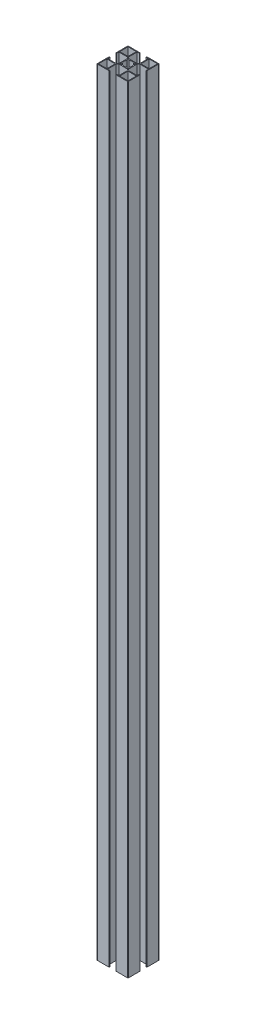
SolidWorks part; units mm, degrees
material "6061 Aluminium alloy"
ref_plane "Front" through (0, 0, 0) normal (0, 0, 1) x (1, 0, 0)
ref_plane "Top" through (0, 0, 0) normal (0, 1, 0) x (1, 0, 0)
ref_plane "Right" through (0, 0, 0) normal (1, 0, 0) x (0, 0, -1)
sketch "Sketch1" plane through (0, 0, 0) normal (0, 1, 0) x (1, 0, 0)
  line L0 (0, 0) -> (0, 20) construction
  line L1 (0, 0) -> (-20, 0) construction
  line L2 (-4.3, 20) -> (-19.5, 20)
  line L3 (-20, 19.5) -> (-20, 4.3)
  line L4 (-20, 4.3) -> (-19.05, 4.3)
  line L5 (-19.05, 4.3) -> (-19.05, 7.25)
  line L6 (-19.05, 7.25) -> (-7.9218, 7.25)
  line L7 (0, 0) -> (-4.3841, 4.3841) construction
  line L8 (-4.3, 20) -> (-4.3, 19.05)
  line L9 (-4.3, 19.05) -> (-7.25, 19.05)
  line L10 (-7.25, 19.05) -> (-7.25, 7.9218)
  line L11 (-7.25, 7.9218) -> (-5.5282, 6.2)
  line L12 (-8.2, 19.05) -> (-19.05, 19.05)
  line L13 (-19.05, 19.05) -> (-19.05, 8.2)
  line L14 (-19.05, 8.2) -> (-8.2, 8.2)
  line L15 (-7.9218, 7.25) -> (-6.2, 5.5282)
  line L16 (-8.2, 19.05) -> (-8.2, 8.2)
  line L17 (-5.5282, 6.2) -> (0, 6.2)
  line L18 (-6.2, 5.5282) -> (-6.2, 0)
  line L19 (-5.0912, 3.677) -> (-4.3875, 2.9732)
  line L20 (-3.677, 5.0912) -> (-2.9732, 4.3875)
  line L21 (0, 6.2) -> (0, 5.3)
  line L22 (-5.3, 0) -> (-6.2, 0)
  arc A0 (-4.3875, 2.9732) -> (-5.3, 0) centre (0, 0) ccw
  arc A1 (-19.5, 20) -> (-20, 19.5) centre (-19.5, 19.5) ccw
  circle A2 centre (0, 0) radius 7.2 construction
  arc A3 (-3.677, 5.0912) -> (-5.0912, 3.677) centre (-4.3841, 4.3841) ccw
  arc A4 (0, 5.3) -> (-2.9732, 4.3875) centre (0, 0) ccw
  dimension "D1" = 10.6
  dimension "D5" = 0.5
  dimension "D17" = 14.4
  dimension "D18" = 2
  dimension "D2" = 40
  dimension "D3" = 40
  dimension "D4" = 8.6
  dimension "D6" = 0.95
  dimension "D7" = 8.6
  dimension "D8" = 14.5
  dimension "D9" = 0.95
  dimension "D10" = 0.95
  dimension "D11" = 0.95
  dimension "D12" = 0.95
  dimension "D13" = 14.5
  dimension "D14" = 13.8
  dimension "D15" = 45
  dimension "D16" = 13.8
extrude "Boss-Extrude1" add sketch "Sketch1" along normal blind 1000
mirror "Mirror1" about plane through (0, 0, 0) normal (1, 0, 0) of "Boss-Extrude1"
mirror "Mirror2" about plane through (0, 0, 0) normal (0, 0, 1) of "Mirror1", "Boss-Extrude1"
